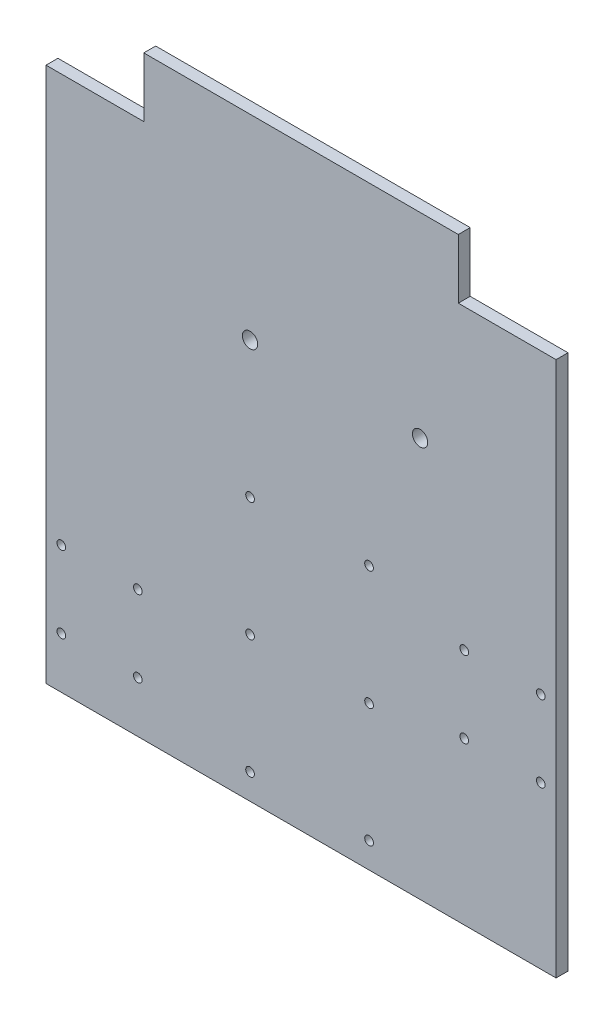
SolidWorks part; units mm, degrees
material "普通碳钢"
ref_plane "前视基准面" through (0, 0, 0) normal (0, 0, 1) x (1, 0, 0)
ref_plane "上视基准面" through (0, 0, 0) normal (0, 1, 0) x (1, 0, 0)
ref_plane "右视基准面" through (0, 0, 0) normal (1, 0, 0) x (0, 0, -1)
sketch "草图1" plane through (0, 0, 0) normal (0, 0, 1) x (1, 0, 0)
  line L0 (115, 700) -> (115, 630)
  line L1 (0, 0) -> (600, 0)
  line L2 (0, 0) -> (0, 630)
  line L3 (115, 700) -> (485, 700)
  line L4 (600, 0) -> (600, 630)
  line L5 (115, 630) -> (0, 630)
  line L6 (485, 700) -> (485, 630)
  line L7 (485, 630) -> (600, 630)
  circle A2 centre (440, 470) radius 9
  circle A3 centre (240, 470) radius 9
  dimension "D6" = 18
  dimension "D1" = 370
  dimension "D2" = 115
  dimension "D3" = 600
  dimension "D4" = 700
  dimension "D5" = 630
  dimension "D8" = 200
  dimension "D9" = 160
  dimension "D10" = 470
extrude "凸台-拉伸1" add sketch "草图1" along normal blind 14
hole_wizard "M12 螺纹孔1" positions "3D草图2" profile "草图3" tap size "M12" standard "GB" end condition through all
sketch3d "3D草图2"
  line L4 (18, 150, 14) -> (108, 150, 14) construction
  line L5 (108, 150, 14) -> (108, 60, 14) construction
  line L6 (108, 60, 14) -> (18, 60, 14) construction
  line L8 (240, 310, 14) -> (240, 30, 14) construction
  line L9 (240, 30, 14) -> (380, 30, 14) construction
  line L10 (380, 30, 14) -> (380, 310, 14) construction
  line L12 (582, 280, 14) -> (582, 190, 14) construction
  line L13 (582, 190, 14) -> (492, 190, 14) construction
  line L14 (492, 190, 14) -> (492, 280, 14) construction
  line L16 (240, 170, 14) -> (380, 170, 14) construction
  line L19 (0, 0, 14) -> (600, 0, 14) construction
  line L20 (0, 630, 14) -> (0, 0, 14) construction
  point P0 (18, 150, 14)
  point P2 (108, 150, 14)
  point P4 (18, 60, 14)
  point P6 (108, 60, 14)
  point P8 (492, 280, 14)
  point P10 (582, 280, 14)
  point P12 (492, 190, 14)
  point P14 (582, 190, 14)
  point P16 (240, 310, 14)
  point P18 (380, 310, 14)
  point P20 (240, 170, 14)
  point P22 (380, 170, 14)
  point P24 (240, 30, 14)
  point P26 (380, 30, 14)
  dimension "D14" = 240
  dimension "D2" = 140
  dimension "D3" = 132
  dimension "D4" = 112
  dimension "D5" = 60
  dimension "D6" = 190
  dimension "D7" = 90
  dimension "D8" = 90
  dimension "D9" = 90
  dimension "D10" = 90
  dimension "D11" = 30
  dimension "D12" = 140
  dimension "D13" = 280
sketch "草图3" plane through (18, 150, 14) normal (1, 0, 0) x (0, -1, 0)
  line L0 (0, 0) -> (0, 14)
  line L1 (0, 14) -> (5.1, 14)
  line L2 (5.1, 14) -> (5.1, 0)
  line L5 (5.1, 0) -> (0, 0)
  line L11 (0, -6.35) -> (0, 107.95) construction
  dimension "通孔螺纹孔钻头直径" = 10.2
  dimension "通孔螺纹孔钻头深度" = 14
cosmetic thread "孔螺蚊线1"
cosmetic thread "孔螺蚊线2"
cosmetic thread "孔螺蚊线3"
cosmetic thread "孔螺蚊线4"
cosmetic thread "孔螺蚊线5"
cosmetic thread "孔螺蚊线6"
cosmetic thread "孔螺蚊线7"
cosmetic thread "孔螺蚊线8"
cosmetic thread "孔螺蚊线9"
cosmetic thread "孔螺蚊线10"
cosmetic thread "孔螺蚊线11"
cosmetic thread "孔螺蚊线12"
cosmetic thread "孔螺蚊线13"
cosmetic thread "孔螺蚊线14"
